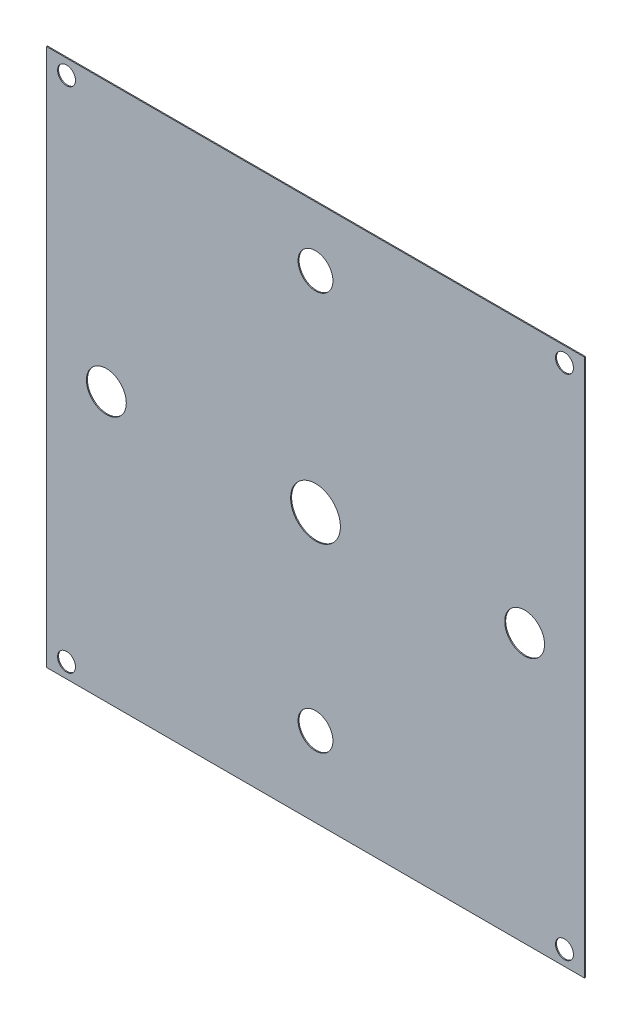
SolidWorks part; units mm, degrees
ref_plane "前视基准面" through (0, 0, 0) normal (0, 0, 1) x (1, 0, 0)
ref_plane "上视基准面" through (0, 0, 0) normal (0, 1, 0) x (1, 0, 0)
ref_plane "右视基准面" through (0, 0, 0) normal (1, 0, 0) x (0, 0, -1)
sketch "草图1" plane through (0, 0, 0) normal (0, 0, 1) x (1, 0, 0)
  line L1 (-270, 270) -> (270, 270)
  line L2 (-270, 270) -> (-270, -270)
  line L3 (-270, -270) -> (270, -270)
  line L4 (270, 270) -> (270, -270)
  line L5 (-270, 270) -> (270, -270) construction
  line L6 (-270, -270) -> (270, 270) construction
  point P0 (0, 0)
  dimension "D1" = 540
  dimension "D2" = 540
extrude "凸台-拉伸1" add sketch "草图1" along normal blind 1
sketch "草图2" plane through (0, 0, 0) normal (0, 0, -1) x (-1, 0, 0)
  circle A0 centre (250, -255) radius 9
  circle A1 centre (-250, -255) radius 9
  circle A2 centre (250, 255) radius 9
  circle A3 centre (-250, 255) radius 9
  dimension "D1" = 18
  dimension "D2" = 18
extrude "切除-拉伸1" cut sketch "草图2" against normal through all
sketch "草图3" plane through (0, 0, 1) normal (0, 0, 1) x (1, 0, 0)
  line L0 (-270, 270) -> (-270, -270) construction
  line L1 (270, -270) -> (270, 270) construction
  circle A0 centre (-210, 0) radius 20
  circle A1 centre (210, 0) radius 20
  dimension "D1" = 40
  dimension "D2" = 40
  dimension "D3" = 60
  dimension "D4" = 60
extrude "切除-拉伸2" cut sketch "草图3" against normal through all
sketch "草图4" plane through (0, 0, 1) normal (0, 0, 1) x (1, 0, 0)
  circle A0 centre (0, 0) radius 25
  dimension "D1" = 50
extrude "切除-拉伸3" cut sketch "草图4" against normal blind 10
sketch "草图5" plane through (0, 0, 0) normal (0, 0, -1) x (-1, 0, 0)
  circle A0 centre (0, -190) radius 17.5
  circle A1 centre (0, 210) radius 17.5
  dimension "D1" = 35
  dimension "D2" = 35
extrude "切除-拉伸4" cut sketch "草图5" against normal through all
